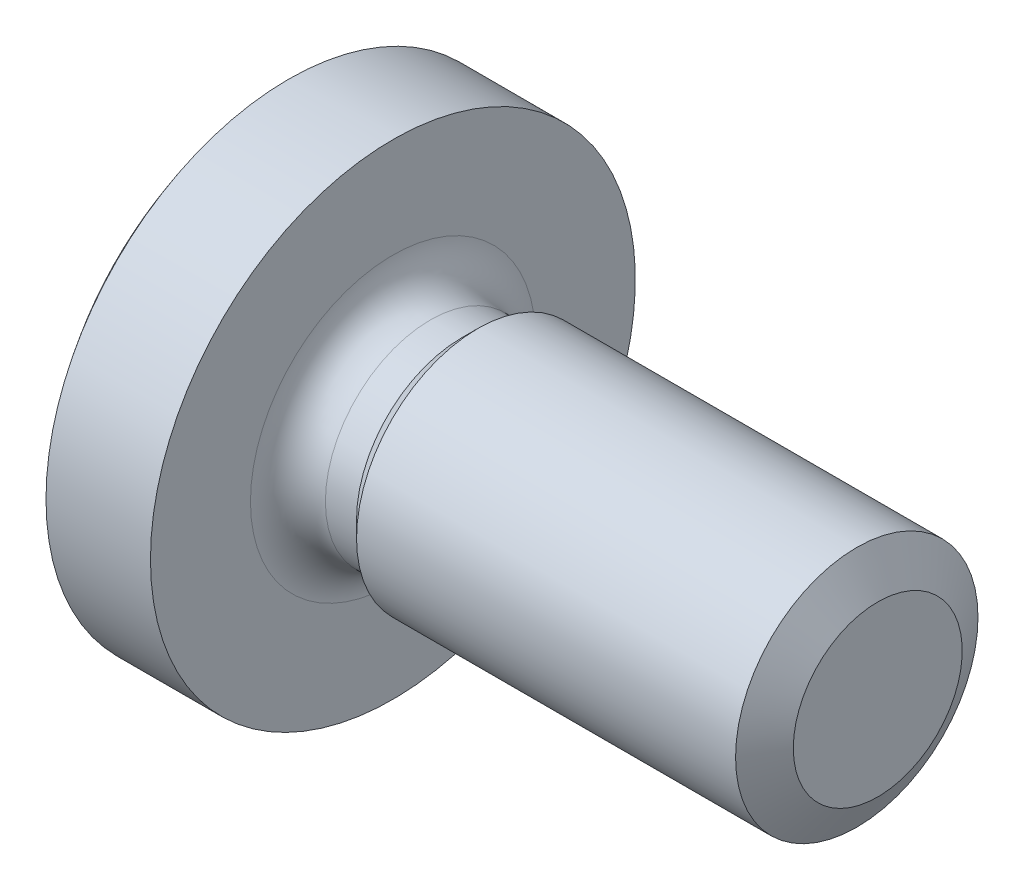
SolidWorks part; units mm, degrees
revolve "Base-Revolve" add sketch "Sketch2" angle 360 about L0
sketch "Sketch2" plane through (0, 0, 0) normal (0, 0, 1) x (1, 0, 0)
  line L0 (-1.3318, 0) -> (6.5885, 0) construction
  line L1 (0, 0) -> (11.1, 0)
  line L2 (11.1, 0) -> (11.1, 2)
  line L3 (11.1, 2) -> (4.5, 2)
  line L4 (4.5, 2) -> (4.232, 1.732)
  line L5 (4.232, 1.732) -> (3.718, 1.732)
  line L6 (3.1, 2.35) -> (3.1, 4)
  line L7 (3.1, 4) -> (1.3765, 4)
  arc A0 (3.1, 2.35) -> (3.718, 1.732) centre (3.718, 2.35) ccw
  arc A1 (0, 0) -> (1.3765, 4) centre (6.5, 0) cw
cosmetic thread "Cosmetic Thread1" parameters "D1"=6.6, "D2"=3.464
ref_plane "Front Plane" through (0, 0, 0) normal (0, 0, 1) x (1, 0, 0)
ref_plane "Top Plane" through (0, 0, 0) normal (0, 1, 0) x (1, 0, 0)
ref_plane "Right Plane" through (0, 0, 0) normal (1, 0, 0) x (0, 0, -1)
sketch "Dimension Sketch" plane through (0, 0, 0) normal (0, 0, 1) x (1, 0, 0)
  line L0 (0, 0) -> (8, 0)
  line L1 (0, 0) -> (0, 8)
  line L2 (8, 0) -> (8, 4.7)
  point P5 (0, 4)
  point P6 (7.3, 0)
  point P7 (1.4, 0)
  point P8 (3.1, 0)
  point P9 (1.5, 0)
  point P10 (4.4, 0)
  point P11 (5.6, 0)
sketch "Sketch3" plane through (0, 0, 0) normal (0, 0, 1) x (1, 0, 0)
  line L0 (10.7538, 2) -> (11.4538, 2)
  line L1 (11.4538, 2) -> (11.1, 1.3938)
  line L2 (11.1, 1.3938) -> (10.7538, 2)
  line L3 (11.1, 2) -> (4.5, 2) construction
  line L4 (11.1, -2) -> (11.1, 2) construction
  line L5 (-0.2428, 0) -> (7.1644, 0) construction
  line L6 (-1.3318, 0) -> (6.5885, 0) construction
revolve "Cut-Revolve1" cut sketch "Sketch3" angle 360 about L5
sketch "Sketch5" plane through (0, 0, 0) normal (1, 0, 0) x (0, 0, -1)
  line L1 (0.35, 2.2) -> (-0.35, 2.2)
  line L2 (0.35, 2.2) -> (0.35, -2.2)
  line L3 (0.35, -2.2) -> (-0.35, -2.2)
  line L4 (-0.35, 2.2) -> (-0.35, -2.2)
  point P4 (0.35, 0)
  point P5 (0, 2.2)
ref_plane "Plane1" through (2.4, 0, 0) normal (1, 0, 0) x (0, 0, -1)
pattern_linear "LPattern1" [suppressed] count 10 spacing 0.7 along (1, 0, 0)
sketch "Sketch6" plane through (2.4, 0, 0) normal (1, 0, 0) x (0, 0, -1)
  point P0 (0, 0)
loft "Cut-Loft1" cut profiles "Sketch6", "Sketch5"
ref_plane "Plane2" through (0, 0, 0) normal (0, -0.7071, 0.7071) x (1, 0, 0)
mirror "Mirror1" about plane through (0, 0, 0) normal (0, -0.7071, 0.7071) of "Cut-Loft1"
equation "\"l@Sketch2\" = \"l@Dimension Sketch\""
equation "\"dk@Sketch2\" = \"dk@Dimension Sketch\""
equation "\"k@Sketch2\" = \"k@Dimension Sketch\""
equation "\"D2@Sketch2\" = \"d@Dimension Sketch\"*0.866"
equation "\"a@Sketch2\" = \"a@Dimension Sketch\""
equation "\"D3@Sketch2\" = \"rf@Dimension Sketch\""
equation "\"d@Sketch2\" = \"d@Dimension Sketch\""
equation "\"da@Sketch2\" = \"da@Dimension Sketch\""
equation "\"D2@Cosmetic Thread1\" = \"d@Dimension Sketch\"*0.866"
equation "\"D1@Cosmetic Thread1\" = \"l@Dimension Sketch\"-\"a@Dimension Sketch\""
equation "\"P@Sketch3\" = \"P@Dimension Sketch\""
equation "\"D1@Sketch3\" = \"P@Dimension Sketch\"*0.866"
equation "\"h@Plane1\" = \"h@Dimension Sketch\""
equation "\"D1@Sketch5\" = \"P@Dimension Sketch\""
equation "\"m@Sketch5\" = \"m@Dimension Sketch\""
equation "\"D3@LPattern1\" = \"P@Dimension Sketch\""
equation "\"D1@LPattern1\" = (\"l@Dimension Sketch\"-\"a@Dimension Sketch\")/\"P@Dimension Sketch\"+1"
